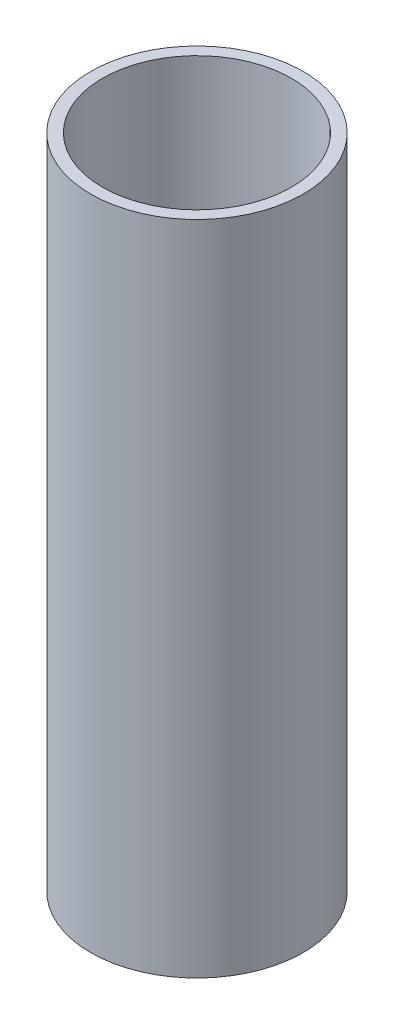
SolidWorks part; units mm, degrees
ref_plane "Front Plane" through (0, 0, 0) normal (0, 0, 1) x (1, 0, 0)
ref_plane "Top Plane" through (0, 0, 0) normal (0, 1, 0) x (1, 0, 0)
ref_plane "Right Plane" through (0, 0, 0) normal (1, 0, 0) x (0, 0, -1)
sketch "Sketch1" plane through (0, 0, 0) normal (0, 1, 0) x (1, 0, 0)
  circle A0 centre (0, 0) radius 450
  circle A1 centre (0, 0) radius 400
  dimension "D1" = 900
  dimension "D2" = 800
extrude "Boss-Extrude1" add sketch "Sketch1" along normal mid plane 3300
sketch "Sketch2" plane through (0, -1650, 0) normal (0, -1, 0) x (1, 0, 0)
  line L0 (0, 0) -> (556.8944, 0)
other "Move Face1" face at (0, -1650, 450) parameters "D1"=518
